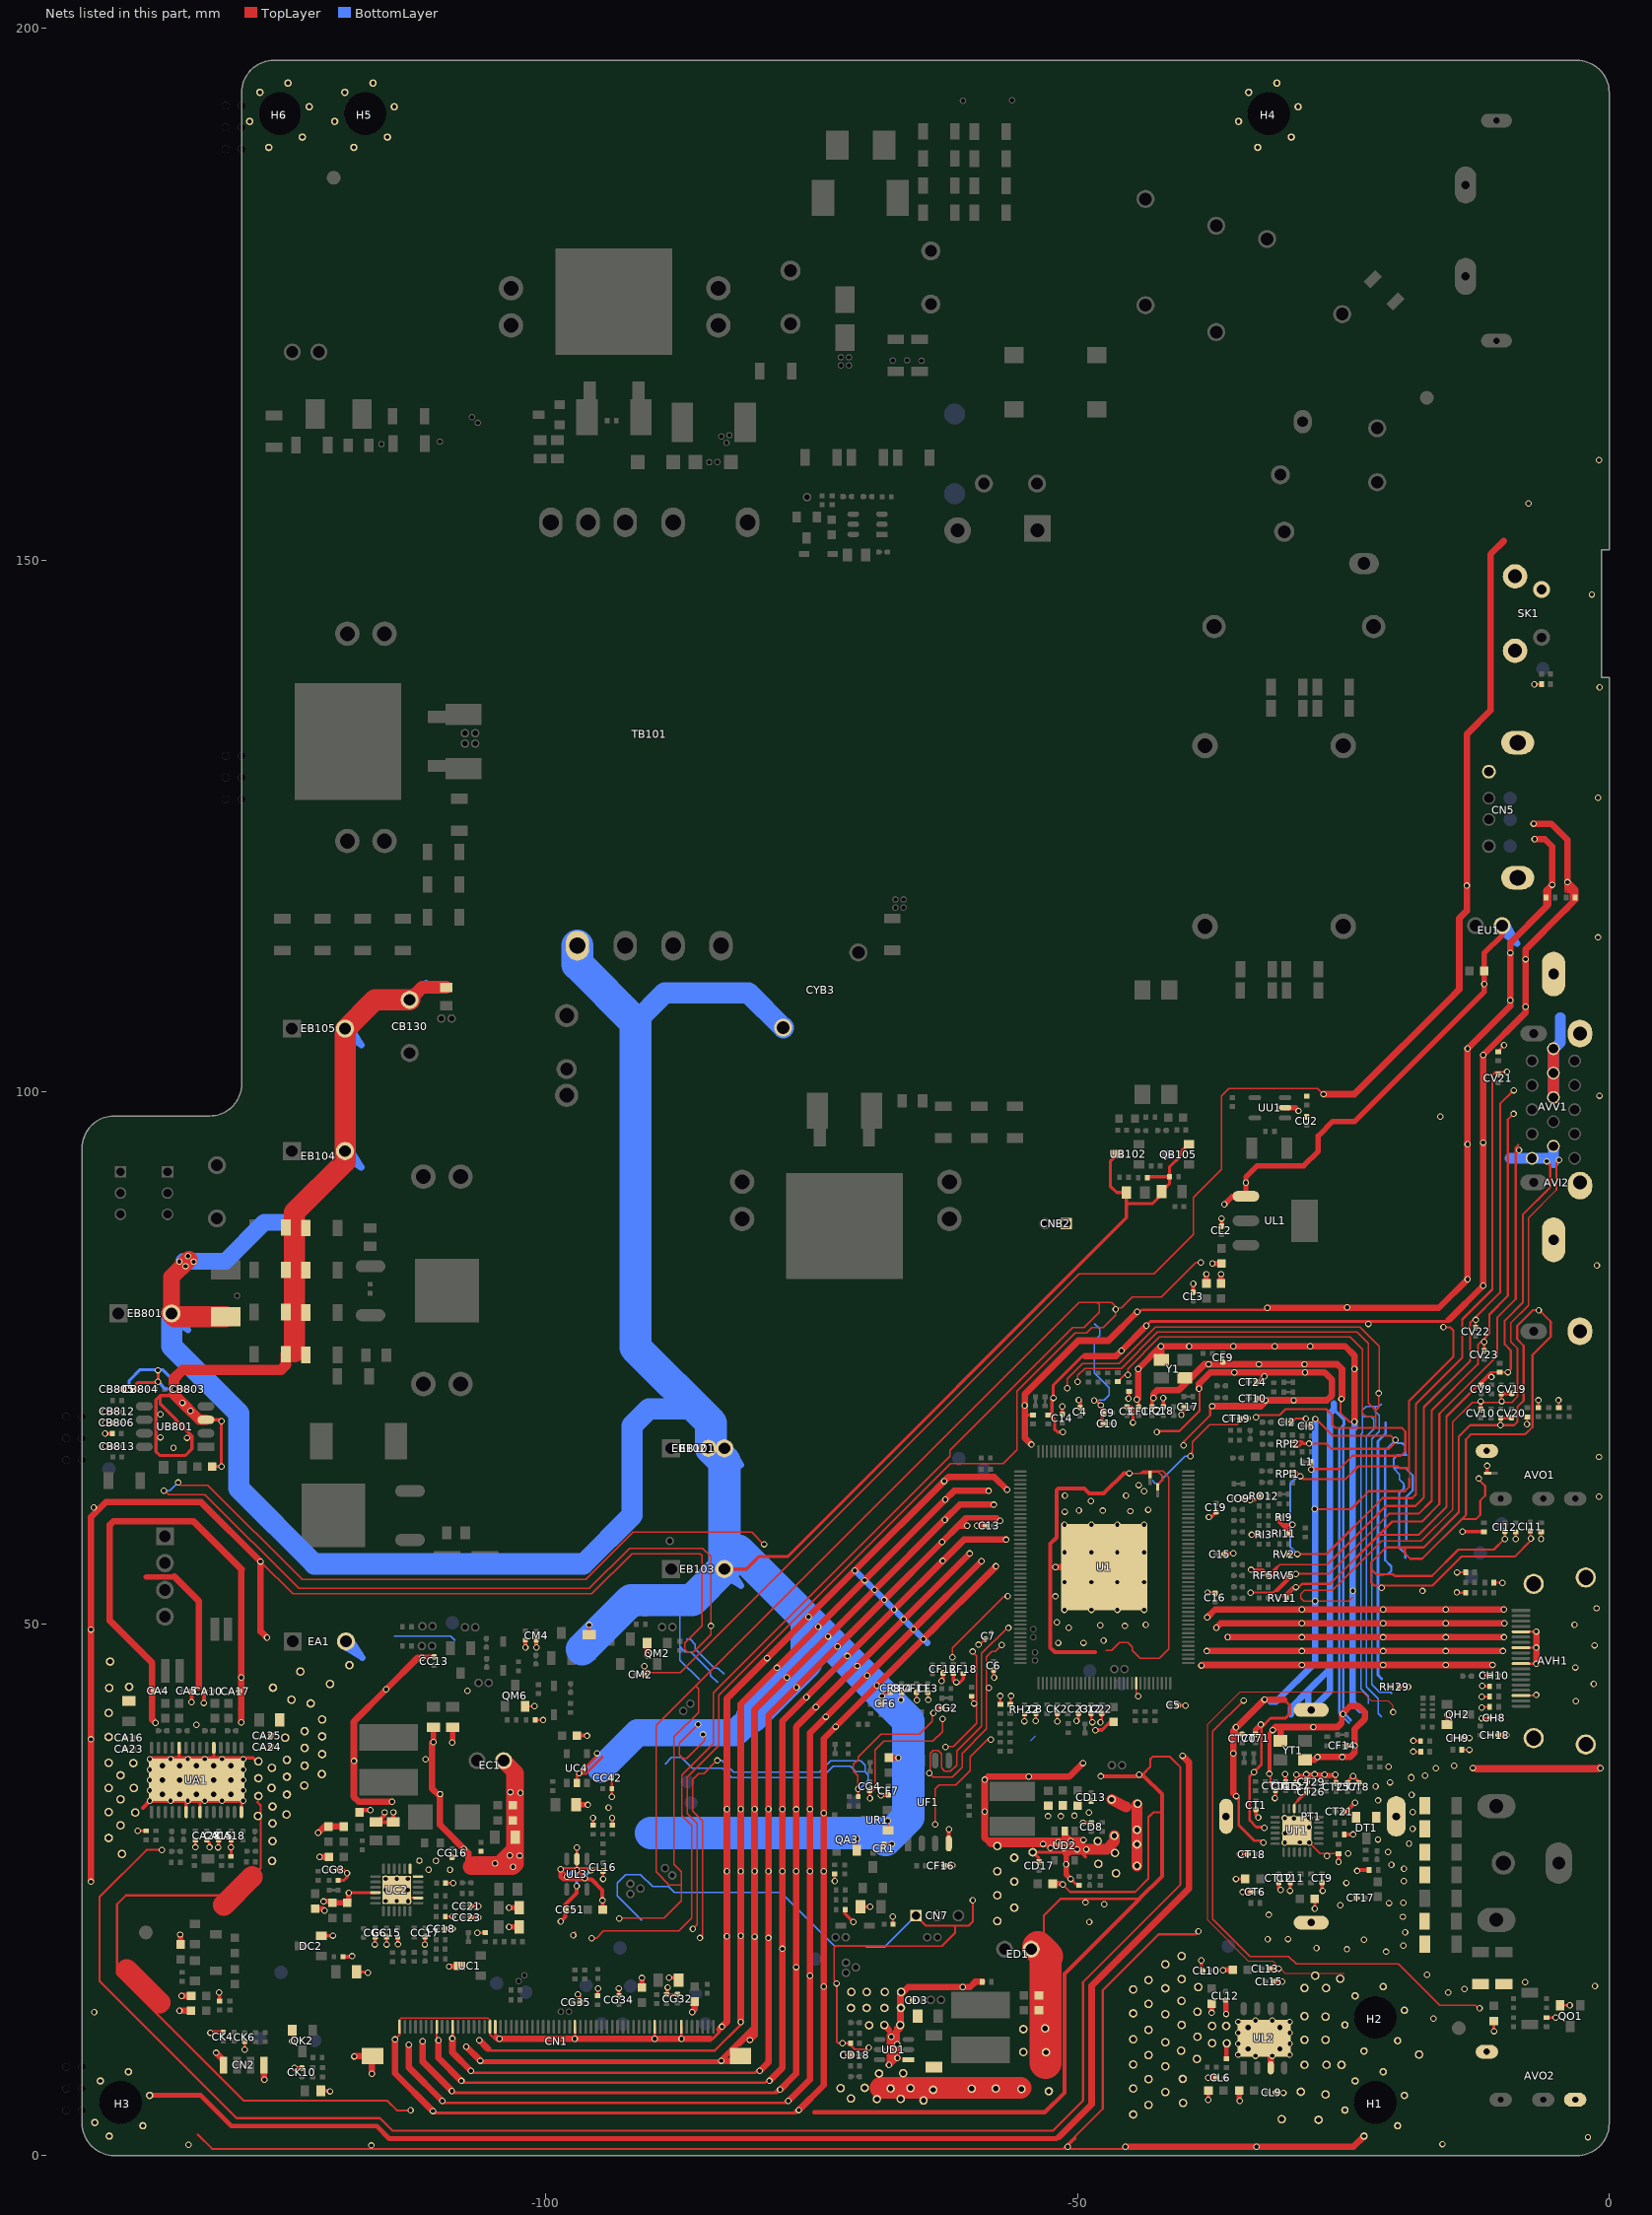
[diagram p0: the nets of this part, all layers, seen from the top]
# Altium PCB MISC86383-9.PcbDoc (part 11 of 18)
Units mm, origin at the board's own origin, x right, y up, seen from the top; angles counter-clockwise.
Board outline 143.6 x 197 mm, 2 copper layers (TopLayer, BottomLayer), stack 1.571 mm thick; 743 components, 401 nets, 2996 pads, 1077 vias.
Unrouted connection lines stored in the file: 4.

## Via types
v1: diameter 0.6, hole 0.4, TopLayer to BottomLayer, tented both sides, 993 vias
v2: diameter 0.6, hole 0.4, TopLayer to BottomLayer, 65 vias
v3: diameter 0.7, hole 0.5, TopLayer to BottomLayer, tented both sides, 15 vias
v4: diameter 0.8, hole 0.5, TopLayer to BottomLayer, tented both sides, 4 vias

## Nets (pads, with @x,y where several pads share a name; then routed paths per layer and width w, separated by ;. In a path a pad name is that pad's centre, name@x,y a point inside that pad or via, vN(x,y) a via of type N, cw(c..) or ccw(c..) an arc to the next point about the centre after c; other vN are vias at no path point) (continued)
GND: (continued)
  TopLayer w0.381: -137.877,32.7 -137.214,33.362 -133.82,33.362 -132.52,33.362 v1(-128.452,33.362) ; v1(-133.332,42.631) -133.314,42.65 CA5.2@-133.314,43.673 ; v1(-132.177,42.555) -132.157,42.574 CA10.2@-132.157,43.66 ; v1(-131.545,11.551) -131.497,11.599 CK4.2@-130.333,11.599 ; RC24.1@-119.082,18.694 -118.262,18.694 v1(-118.212,18.745) ; CG14.2@-117.5,32.266 -117.292,32.474 v1(-116.51,32.474) ; v1(-115.151,32.271) -115.151,32.017 -115.809,31.359 RG58.2@-115.976,31.359 RG63.2@-114.351,31.359 -114.351,32.042 -114.338,32.055 v1(-114.338,32.271) ; v1(-111.62,46.812) -111.513,46.92 CC13.1@-110.503,46.92 ; v1(-106.15,8.907) -106.036,8.793 -83.611,8.793 v1(-83.496,8.907) -81.912,10.491 ; v1(-101.917,47.765) RM6.2@-101.917,48.445 ; CM4.2@-100.902,48.444 -100.902,47.777 v1(-100.889,47.765) ; v1(-98.606,26.904) -98.606,26.205 -98.359,25.958 -95.688,25.958 -94.678,24.948 v1(-94.678,23.978) -94.678,23.939 -94.645,23.906 CC50.2@-94.645,23.114 ; v1(-98.59,22.009) -98.164,22.435 CC51.1@-98.164,23.114 -98.164,23.609 -97.097,24.676 v1(-97.097,25.353) ; CC38.1@-97.071,39.484 -96.152,39.484 v1(-96.126,39.459) ; -74.778,4.069 -53.065,4.069 -51.224,5.909 -51.224,17.087 -44.181,24.13 ; CF16.2@-62.458,27.254 -61.804,27.254 v1(-61.766,27.292) ; UF1.4@-62.106,29.342 -62.106,30.629 v1(-62.078,30.658) ; -48.355,47.327 -52.121,47.327 -52.546,47.752 -52.546,57.526 -51.964,58.108 -51.964,62.563 -51.797,62.729 -49.373,62.729 -48.888,62.244 -47.538,62.244 -45.63,64.152 v1(-45.109,64.152) ; v1(-47.803,35.662) -43.752,35.662 ; v1(-44.194,35.808) -43.899,35.808 -43.891,35.801 -43.752,35.662 ; -44.162,24.149 -42.056,26.255 -42.056,32.258 -42.056,33.965 -43.752,35.662 ; -43.415,35.325 -43.752,35.662 ; CL3.1@-39.116,81.197 v2(-39.116,81.966) ; v1(-37.719,7.315) CL6.1@-36.975,7.315 ; v1(-37.694,5.232) -37.689,5.237 CL7.1@-37.689,6.096 ; CL2.1@-36.449,87.416 v2(-36.449,88.113) ; RL4.1@-35.992,9.112 -35.992,10.515 pad.VIA5@-35.966,10.54 ; CT70.2@-34.55,39.66 CT70.2@-34.52,39.629 ; v2@-31.954,35.775 -31.954,39.703 v1(-31.65,40.007) ; CL15.2@-31.528,16.358 v1(-30.759,16.358) ; RI9.1@-31.002,59.921 -31.002,59.571 -30.633,59.203 ; v1@-30.915,24.976 v1@-30.871,24.932 ; RI11.1@-30.152,58.486 -30.152,58.721 -30.633,59.203 ; v1(-30.007,24.894) v1@-29.987,24.914 ; v1(-29.791,59.307) -30.529,59.307 -30.633,59.203 ; v1@-29.436,35.765 -29.368,35.698 v1@-28.451,35.698 ; CT29.1@-28.451,35.13 v1@-28.451,35.698 ; -26.26,35.666 -27.213,35.666 -27.245,35.698 -25.859,35.698 v1(-25.753,35.803) v1(-26.782,35.803) ; v1@-25.435,27.726 LT6.2@-25.435,28.393 ; v1@-25.327,23.564 -25.313,23.564 v1(-25.284,23.536) ; CT21.2@-24.947,32.348 -24.719,32.348 v1(-23.883,33.185) ; LT8.2@-24.921,30.177 v1@-24.089,30.177 ; CF14.1@-24.685,38.547 -23.954,38.547 v1(-23.941,38.534) ; v1(-23.695,26.761) -23.618,26.838 LT11.2@-22.571,26.838 ; v1@-1.155,83.62 v1(-1.155,83.679) ; v1@-0.973,65.633 -0.973,65.668 v1(-0.955,65.686) ; v1@-28.451,35.698 -27.958,35.698 -27.852,35.803 v1(-26.782,35.803) ; v1@-28.451,35.698 -28.451,35.822 v1(-28.471,35.841) v1(-27.696,35.841) -26.82,35.841 v1(-26.782,35.803)
  TopLayer w0.457: H3.4@-137.25,5.65 -132.445,5.65 -129.564,2.769 ; -128.727,2.769 -129.564,2.769 ; -51.675,1.906 -51.989,1.592 -114.725,1.592 -115.901,2.769 -129.564,2.769 ; -49.398,75.163 -49.29,75.163
  TopLayer w0.508: -137.594,54.421 -134.914,54.421 -134.125,53.632 ; v1(-134.379,20.777) -134.353,20.752 CG28.2@-134.353,19.845 ; CC5.2@-121.672,23.213 -121.015,23.213 v1(-120.82,23.017) ; v1@-120.905,23.877 v1(-120.905,23.886) -120.182,23.886 CC7.1@-120.053,23.757 CC4.2@-118.681,23.757 ; CC4.2@-118.686,23.762 CC4.2@-118.681,23.757 ; v1(-118.516,24.701) -118.516,23.922 CC4.2@-118.594,23.845 ; CC12.1@-110.582,40.253 -110.582,38.891 v1(-110.579,38.887) ; v1(-109.106,17.763) -109.034,17.763 -109.03,17.768 -108.179,17.768 UC1.3@-108.103,17.843 ; v1(-108.814,38.824) -108.75,38.824 -108.75,40.25 CC8.1@-108.753,40.253 ; v1@-103.454,21.483 CC1.1@-102.488,21.483 ; v1@-103.454,23.312 CC2.1@-102.488,23.312 ; CC43.1@-97.154,32.982 -96.05,32.982 v1(-96.037,32.969) ; CG33.1@-90.957,15.794 v1(-90.957,16.7) ; QM2.E@-90.475,48.197 -90.475,47.066 v1(-90.437,47.028) ; CF10.1@-67.755,37.41 -66.856,37.41 v1(-66.84,37.395) ; -60.533,59.893 -60.482,59.945 -57.604,59.945 -57.302,59.643 -57.252,59.643 v1(-57.252,59.69) ; CD16.1@-52.329,25.552 -51.46,25.552 v1(-51.384,25.476) ; v1(-50.648,26.01) -51.073,26.435 v1(-51.073,27.366) -51.073,28.402 -50.959,28.516 -50.936,28.538 -49.791,28.538 ; CL5.1@-37.871,82.004 v2(-37.871,82.88) ; v1(-37.389,13.411) CL11.2@-37.389,14.28 ; v2(-37.313,83.871) -37.308,83.876 CL1.1@-36.449,83.876 ; CL4.1@-36.5,82.004 v2(-36.5,82.88) ; v1(-36.322,17.424) -36.271,17.475 CL14.2@-35.403,17.475 ; v2(-36.195,89.433) -35.43,90.198 UL1.1@-34.163,90.198 v2(-34.163,91.491) -34.163,91.999 -33.096,93.066 -28.727,93.066 -27.356,94.437 -27.356,94.945 ; v1(-36.017,13.31) -36.017,14.28 ; -35.138,39.66 -35.138,40.144 v1@-35.138,40.214 ; v1@-35.092,40.342 v1(-35.092,40.26) ; CL8.1@-34.793,6.096 -34.793,5.177 v1(-34.747,5.131) ; CT71.1@-33.266,39.654 -33.266,40.045 -33.251,40.045 v1(-32.768,40.528) ; CL13.2@-31.884,17.577 v1(-31.09,17.577) ; UU1.2@-30.477,98.527 -29.515,98.527 v1(-29.21,98.222) ; -27.356,95.484 -27.356,94.945 ; -25.205,40.622 -25.154,40.672 -25.154,41.401 v1(-25.035,41.52) ; v2@-11.74,110.165 CU1.1@-11.74,111.379 ; EU1.2@-10.078,115.646 -10.078,114.737 -11.735,113.081 v2(-11.735,110.16) -11.735,109.436 -23.94,97.231 -25.997,97.231 -27.356,95.872 -27.356,94.945 ; -4.411,116.87 -4.376,116.87 -3.392,117.853 ; -4.411,116.871 -4.411,116.942 -3.392,117.961 DU4.A@-3.199,118.154 ; CC4.2@-118.681,23.757 CC4.2@-118.594,23.845 ; CC4.2@-118.681,23.757 -118.681,23.845 CC4.2@-118.594,23.845 ; v1@-35.138,40.214 v1(-35.092,40.26) ; v1@-35.138,40.214 -35.138,40.26 v1(-35.092,40.26)
  TopLayer w0.61: v1(-142.775,25.742) v1(-142.775,39.132) v1(-142.775,49.462) -142.775,60.033 -141.377,61.43 -132.41,61.43 v2(-126.835,55.854) -126.835,49.314 ; -140.997,51.15 -140.997,50.293 ; v1(-136.711,40.675) -137.015,40.98 -137.015,46.312 -140.997,50.293 ; -134.937,54.445 -134.914,54.421 -132.639,52.146 -132.639,44.044 ; v1(-134.455,13.614) CC34.1@-133.358,13.614 ; v1(-134.239,15.011) CC33.1@-133.345,15.011 ; v1(-131.009,9.659) -130.305,8.955 CN2.1@-130.305,8.505 CN2.1@-130.289,8.489 ; v1@-128.638,44.955 -128.638,48.59 ; -128.638,47.284 -128.638,48.59 ; v1(-128.633,40.739) v1(-128.633,44.955) ; -128.613,55.118 -129.673,56.178 ; -126.835,49.276 -126.835,49.314 ; CN2.4@-126.495,8.505 -126.495,7.153 v1(-126.467,7.125) ; v1(-126.213,48.692) -126.835,49.314 ; v1(-121.4,30.34) -120.807,30.932 CC10.2@-120.421,30.932 CC9.2@-118.999,30.932 ; v1(-121.26,28.08) -121.094,28.08 -121.082,28.092 CC11.2@-120.404,28.092 ; v1(-118.008,9.322) -117.978,9.353 CN1.62@-116.29,9.353 -116.357,9.285 v1(-116.357,7.671) ; v1(-114.449,33.261) -117.593,33.261 -118.046,33.715 v1(-118.046,37.097) -118.046,40.793 v1(-115.015,43.825) -112.028,46.812 v1(-111.62,46.812) ; v1(-114.173,10.909) v1(-114.173,10.909) -114.172,7.733 v1(-110.622,4.183) ; v1(-112.871,10.414) -112.871,8.272 v1(-109.727,5.128) ; v1(-111.571,10.757) -111.571,8.81 v1(-108.833,6.073) ; v1@-110.582,38.891 -110.718,38.755 -110.718,34.519 -109.969,33.77 -109.969,31.102 -107.29,28.423 -107.29,27.826 ; v1(-110.084,10.82) -110.084,9.162 v1(-107.939,7.018) ; v1@-108.783,11.024 v1(-108.783,11) -108.783,9.701 v1(-107.044,7.962) ; v1(-107.483,10.24) v1(-106.15,8.907) ; v1(-106.241,10.837) -105.432,10.028 ; -104.681,11.116 -104.537,10.973 v1(-104.343,10.973) v1(-97.282,10.973) v1(-89.764,10.973) v1(-87.236,10.973) -84.57,10.973 ; v1(-86.246,13.487) -85.992,13.741 CG31.1@-85.992,14.47 ; -83.693,11.85 v1(-83.431,12.112) -82.969,12.574 v1(-82.969,20.626) v1(-82.969,32.563) -82.969,42.978 v1(-70.931,55.016) v1(-62.535,63.412) -62.15,63.797 -57.816,63.797 v1(-56.624,62.604) ; v1(-83.496,8.907) -82.155,8.907 CN1.61@-81.71,9.353 ; -81.912,10.491 -80.368,12.036 ; v1(-81.668,12.548) v1(-81.668,20.656) -81.668,42.44 v1(-62.433,61.675) -61.611,62.496 v1(-58.355,62.496) ; v1(-80.823,10.858) -80.368,11.314 -80.368,12.036 ; -80.368,21.199 v1(-80.368,20.584) ; -80.368,24.028 -80.368,24.638 ; v1(-79.869,7.962) -79.425,8.407 -79.065,8.767 -79.065,11.716 v1(-79.065,20.455) ; -79.065,21.221 v1(-79.065,20.455) ; v1(-78.975,7.018) -78.785,7.208 -77.765,8.228 -77.765,12.436 ; v1(-77.967,6.187) -76.824,7.33 ; -77.765,13.462 -77.765,12.436 ; -77.765,21.391 v1(-77.765,19.435) ; -77.24,6.914 -76.824,7.33 ; v1@-77.059,5.255 -75.164,7.151 -75.164,17.424 ; -76.464,15.189 -76.464,13.371 ; -76.464,20.665 v1(-76.464,17.715) ; v1(-76.204,4.271) -73.863,6.612 -73.863,14.224 v1(-73.863,15.887) v1(-73.863,32.207) ; -75.164,16.561 v1(-75.164,16.903) -75.164,17.424 ; v1@-73.863,32.41 v1(-73.863,32.207) ; pad.VIA5@-68.17,12.263 -67.721,11.815 ; v1(-67.721,8.519) v1@-67.627,8.613 ; v1@-67.627,11.283 -67.627,10.333 v1@-67.627,8.613 ; v1@-67.618,9.862 v1(-67.607,9.862) ; -66.98,11.361 v1@-66.98,10.508 ; pad.VIA5@-66.624,12.192 -66.65,12.217 -66.65,15.113 -65.913,15.85 v1(-60.782,15.85) ; -63.267,49.803 v1(-64.498,48.572) ; -60.533,59.893 -61.22,59.207 ; v1(-60.361,59.207) -61.22,59.207 ; -60.316,15.826 -60.782,15.826 v1(-60.782,15.85) ; v1(-60.143,56.606) v1(-66.338,50.41) -76.464,40.284 v1(-76.464,17.715) ; v1(-59.02,55.889) v1(-65.41,49.499) -75.164,39.745 -75.164,17.424 ; DK6.A@-58.947,16.332 -59.607,16.332 -60.09,15.85 v1(-60.782,15.85) ; v1(-57.872,61.196) -61.073,61.196 v1(-62.477,59.792) v1(-69.085,53.183) -80.368,41.901 -80.368,24.638 ; v1(-57.667,55.403) v1(-64.498,48.572) ; v1(-56.703,57.906) -60.681,57.906 v1(-62.672,55.916) v1(-67.246,51.341) -77.765,40.823 v1(-77.765,19.435) ; v1(-54.331,66.853) -54.966,67.488 -54.966,69.716 v1(-54.966,70.529) -54.966,71.577 -49.922,76.621 -47.085,76.621 v1(-44.378,79.328) ; v1(-52.07,55.321) -52.062,55.313 U1.157@-47.471,55.313 ; v1(-51.821,29.464) -51.821,29.396 v1@-51.918,29.299 ; -51.731,1.754 -48.672,4.814 -48.672,15.964 -39.503,25.132 -39.503,36.963 v1(-40.132,37.592) ; v1(-51.308,28.905) v1(-50.648,29.566) ; UD2.2@-51.199,30.507 UD2.2@-51.199,30.117 ; v1(-50.038,28.792) v1@-50.038,28.956 ; v1(-49.484,36.898) -50.758,35.623 v1(-54.585,35.623) -58.434,35.623 v1(-58.725,35.332) v1(-58.725,32.334) -58.725,29.867 -58.46,29.603 ; -49.29,75.163 -46.391,75.163 v1(-45.872,75.682) v1(-43.525,78.029) ; v1(-45.494,0.826) v1(-33.172,0.826) -24.049,0.826 H1.6@-23.05,1.825 ; v1(-44.425,71.082) -44.278,71.229 v1@-44.278,73.938 ; v1(-44.296,73.956) v1(-42.168,76.084) v1(-39.497,76.084) v1(-35.344,76.084) v1(-31.458,76.084) v1(-28.118,76.084) -24.814,76.084 -23.96,75.23 v1(-23.96,73.97) v1(-23.96,68.991) ; v1(-42.848,71.213) -42.848,71.607 -42.47,71.985 -40.475,71.985 -38.06,74.401 v1(-37.653,74.401) v1(-32.941,74.401) v1(-28.651,74.401) -25.569,74.401 -25.128,73.959 -25.128,71.2 v1(-25.179,71.15) ; v1@-42.15,76.066 -42.106,76.022 Y1.2@-42.106,74.82 ; v1(-38.568,72.115) -38.568,72.572 -37.501,73.639 v1(-35.255,73.639) v1(-28.602,73.639) -26.75,73.639 -26.06,72.949 -26.06,71.485 -26.53,71.015 v1(-29.667,71.015) v1(-32.343,71.015) -32.343,70.86 -32.744,70.459 v1(-37.327,70.459) ; v1(-38.34,46.079) -38.29,46.129 v1(-28.906,46.129) v1(-21.26,46.129) v1(-15.354,46.129) v1(-10.97,46.129) ; v1(-37.851,47.429) v1(-28.906,47.429) v1(-21.26,47.429) v1(-15.354,47.429) v1(-9.982,47.429) ; v1(-37.814,50.589) -37.066,51.337 v1(-28.906,51.337) v1(-9.892,51.337) ; v1(-36.943,49.622) -36.528,50.037 v1(-28.906,50.037) v1(-21.26,50.037) v1(-15.354,50.037) v1(-9.853,50.037) ; v1(-35.877,48.736) -35.871,48.73 v1(-28.906,48.73) v1(-21.26,48.73) v1(-15.354,48.73) v1(-9.884,48.73) ; v1@-35.138,33.855 -35.352,34.07 -35.352,39.929 -35.138,40.144 v1(-32.404,42.878) -30.574,42.878 ; UL2.EPAD@-32.461,11.024 -31.826,10.389 UL2.3@-31.826,8.241 ; v2(-32.155,79.705) -23.546,79.705 ; v1(-31.65,40.007) -31.369,40.289 v1(-27.815,40.289) -25.537,40.289 -25.205,40.622 ; YT1.4@-30.908,39.002 -30.908,40.18 ; YT1.2@-28.608,37.202 -27.699,37.202 v1(-27.434,37.467) v1(-25.11,37.467) -24.36,37.467 -23.941,37.886 v1(-23.941,38.534) -23.941,40.096 -22.951,41.087 -22.952,41.088 -22.952,41.652 -23.557,42.257 -24.362,42.257 v1@-25.035,41.585 ; v2(-26.873,99.797) -23.96,99.797 -14.723,109.034 ; v1@-25.154,41.401 -25.154,41.466 v1@-25.035,41.585 ; v1(-25.035,41.52) v1@-25.035,41.585 ; v1(-24.638,79.756) -24.587,79.705 -23.546,79.705 ; -15.076,78.577 v1(-11.854,81.799) v1(-11.854,95.25) v1(-11.854,103.475) -7.847,107.481 v1(-7.847,108.024) v1(-7.847,112.493) -7.847,113.398 ; -14.503,109.254 -14.723,109.034 ; -13.995,116.434 -13.392,117.037 ; v2(-13.392,119.405) -13.392,123.215 ; v1(-12.827,36.436) v1@-0.851,36.436 ; CN5.4@-11.31,129.959 CN5.4@-11.31,130.13 ; -9.922,151.807 -11.144,150.585 -11.144,135.889 -13.392,133.641 -13.392,123.215 ; v1(-7.102,125.238) -5.452,125.238 -3.907,123.693 v1(-3.907,119.732) ; v1(-7.007,123.78) -6.056,123.78 -5.365,123.089 v1(-5.365,119.487) -5.736,119.116 ; v1(-6.858,46.228) v1(-6.858,47.752) v1(-6.858,49.276) ; -4.376,116.87 -7.847,113.398 ; -3.864,117.417 -4.097,117.184 ; -3.392,117.961 -3.392,118.761 -3.907,119.275 v1(-3.907,119.732) ; v1@-0.945,36.53 v1@-0.851,36.436 ; v1(-0.826,36.411) v1@-0.851,36.436 ; -140.997,50.293 -140.997,59.296 -140.641,59.652 -133.147,59.652 -129.673,56.178 ; -129.673,56.178 -128.638,55.143 -128.638,48.59 ; -80.368,12.036 -80.368,12.497 v1(-80.368,20.584) ; v1(-80.368,20.584) -80.368,24.638 ; v1(-79.065,20.455) -79.065,41.361 v1(-68.175,52.253) v1(-62.728,57.699) -61.22,59.207 ; -77.765,12.436 v1(-77.765,19.435) ; -76.824,7.33 -76.464,7.689 -76.464,13.371 ; -76.464,13.371 v1(-76.464,17.715) ; v1(-73.863,32.207) -73.863,39.207 v1(-64.498,48.572) ; v1@-67.627,8.613 -67.074,9.166 v1(-66.933,9.166) v1@-66.98,9.213 ; v1(-67.607,9.862) -67.552,9.862 v1@-66.98,10.434 ; v1(-67.607,9.862) -67.607,9.84 v1@-66.98,9.213 ; v1@-66.98,9.213 v1@-66.98,10.434 ; v1@-66.98,10.434 v1@-66.98,10.508 ; v1@-66.98,10.434 v1(-66.943,10.471) v1@-66.98,10.508 ; v1@-66.98,10.508 -67.505,11.034 v1(-67.505,11.157) -66.933,11.73 ; -66.933,11.73 -66.933,11.993 pad.VIA5@-66.663,12.263 -66.663,12 -66.933,11.73 ; -58.46,29.603 -51.257,29.603 ; -58.46,29.603 -58.156,29.299 v1(-53.238,29.299) v1@-51.918,29.299 ; v1@-51.918,29.299 -51.561,29.299 -51.257,29.603 ; -51.257,29.603 -51.199,29.661 ; -51.199,29.661 UD2.2@-51.199,30.117 ; -51.199,29.661 -51.193,29.667 v1@-50.749,29.667 ; UD2.2@-51.199,30.117 v1@-50.749,29.667 ; v1@-50.749,29.667 v1(-49.428,29.667) -50.038,29.058 v1@-50.038,28.956 ; v1@-50.749,29.667 v1(-50.648,29.566) ; v1(-50.648,29.566) v1@-50.038,28.956 ; -23.546,79.705 -16.01,79.705 v1(-13.312,82.403) v1(-13.312,95.098) v1(-13.312,104.078) -9.305,108.085 v1(-9.305,108.628) v1(-9.305,113.097) -9.305,114.037 -5.929,117.413 ; -14.723,109.034 -14.092,109.665 -14.092,116.337 -13.392,117.037 ; -13.392,117.037 -13.392,123.215 ; -7.847,113.398 -7.847,113.433 ; -7.847,113.433 -4.411,116.87 -4.097,117.184 ; -7.847,113.434 -4.411,116.871 -4.097,117.184 ; -5.929,117.413 DU3.A@-5.929,118.305 -5.925,118.309 -5.925,118.927 -5.736,119.116 ; -5.929,117.413 -5.736,117.607 -5.736,119.116 ; -4.097,117.184 -3.199,118.082 -3.199,118.154 DU4.A@-3.199,118.307 -3.199,119.025 v1(-3.907,119.732)
  TopLayer w1: v2(-133.427,70.027) -132.95,69.551 ; UB801.3@-131.961,69.18 -132.58,69.18 -132.95,69.551 ; RB839.2@-124.446,75.349 -124.446,74.347 -124.917,73.876 -134.158,73.876 -134.975,73.059 -134.975,71.576 v2(-134.176,70.777) -132.95,69.551
  TopLayer w1.016: -51.001,28.603 -50.812,28.792 v1(-50.038,28.792) v1(-49.174,28.792) -47.249,28.792 -46.519,29.523 pad.VIA5@-46.533,30.074 ; pad.VIA5@-46.787,33.477 -45.431,32.766 ; pad.VIA5@-44.405,27.228 pad.VIA5@-44.405,29.26 pad.VIA5@-44.405,32.994 ; AVV1.8@-5.247,99.595 AVV1.7@-5.247,101.785 AVV1.6@-5.247,104.075 AVV1.6@-5.247,104.175
  TopLayer w1.2: CB130.1@-112.812,108.661 -111.629,109.845 RB140.2@-109.36,109.845
  TopLayer w1.524: -107.038,27.14 -104.623,27.14 ; -106.718,27.368 -104.394,27.368 ; -104.369,27.368 -104.394,27.368 ; EC1.2@-103.969,37.122 -102.946,36.099 ; -104.623,27.14 pad.VIA5@-103.083,27.14 -102.806,27.417 -102.806,28.956 ; -104.623,27.14 -104.394,27.368 ; -104.394,27.368 -102.946,28.816 ; -102.946,28.816 -102.946,36.099 ; -102.946,28.816 -102.806,28.956 ; -102.946,36.099 -102.806,35.959 -102.806,28.956
  TopLayer w1.6: EB801.2@-135.193,79.184 -135.193,82.599 -133.547,84.245
  TopLayer w2: EB801.2@-135.193,79.184 -134.873,78.864 DB804.K@-130.111,78.864 ; -123.622,75.578 -123.622,88.697 -118.874,93.445 EB104.2@-118.874,94.45 -118.874,105.865 -116.078,108.661 CB130.1@-112.812,108.661
  TopLayer w2.032: -139.396,17.446 -136.324,14.374 ; -130.273,23.546 -130.282,23.546 -127.618,26.209 ; -68.529,6.375 pad.VIA5@-55.334,6.375
  TopLayer w3: ED1.2@-53.726,19.601 -52.996,18.871 ; -52.996,8.714 -52.996,18.871 ; -52.856,18.731 -52.996,18.871
  BottomLayer w0.102: -54.394,39.017 -53.926,39.486
  BottomLayer w0.127: v2(-135.903,62.522) -135.344,62.522 v2(-134.582,63.284) ; -114.267,48.852 -108.948,48.852 -108.509,48.412 ; -90.946,22.084 -93.256,24.393 -93.256,25.627 -92.467,26.416 -91.084,26.416 -89.952,25.284 -88.46,25.284 -87.903,24.727 -77.876,24.727 -72.834,19.685 -69.124,19.685 -69.086,19.647 ; -88.794,36.792 -88.163,37.422 -87.262,37.422 -86.238,36.398 -83.42,36.398 -82.548,35.527 -74.062,35.527 -72.98,36.609 -71.369,36.609 -70.836,36.076 -69.964,36.076 ; -87.404,47.844 -86.923,47.363 -86.381,47.363 -84.501,45.483 -84.501,45.149 -83.845,44.492 ; -86.786,48.54 -86.429,48.54 -85.946,48.057 -85.946,47.646 -84.142,45.842 -83.807,45.842 -83.216,45.251 ; -86.248,52.222 -87.37,51.1 -87.37,46.59 -85.56,44.78 ; v1@-84.066,37.143 -83.446,37.143 -82.338,36.035 -74.273,36.035 -73.19,37.117 -70.366,37.117 -69.964,36.716 -69.964,36.076 ; v1(-70.637,34.468) -70.46,34.468 -69.677,35.25 -69.677,35.789 -69.964,36.076 ; -48.396,78.228 -47.904,77.737 -47.904,77.114 -48.435,76.584 -48.435,73.595 -47.031,72.191 -47.031,71.511 -47.503,71.04 -48.009,71.04 ; -42.954,63.462 -42.717,63.225 -42.331,63.225 -42.059,63.498 -42.059,63.58 -39.878,65.761 v1(-39.383,65.761) ; v1(-23.96,68.991) -23.96,70.362 ; -22.657,42.486 -22.657,43.182 -23.359,43.884 -23.359,61.955 -23.359,67.098 -23.355,67.103 -23.355,67.796 -23.185,67.966 -23.185,69.435 ; -21.412,70.675 -21.654,70.434 -21.978,70.434 ; -21.386,41.247 -21.714,41.575 -21.714,42.957 -22.83,44.073 -22.83,67.603 -22.136,68.296 -22.136,69.219 -22.36,69.443 -23.178,69.443 -23.185,69.435 ; -20.401,43.41 -20.542,43.552 -21.59,43.552 -22.322,44.283 -22.322,67.392 -21.628,68.086 -21.628,69.58 -21.978,69.93 -21.978,70.434 ; -20.252,64.727 -20.252,64.59 -19.715,64.054 -19.715,63.567 -19.313,63.165 -19.313,62.992 ; -23.185,69.435 -23.185,70.091 -22.842,70.434 -21.978,70.434
  BottomLayer w0.203: -69.85,19.647 -69.086,19.647 -68.104,19.647 CN7.1@-65.195,22.555 ; v1(-29.307,56.552) -30.001,57.245 -30.001,63.151 -29.281,63.871 v1(-29.053,63.871) ; -25.062,68.581 -25.379,68.264 -25.379,41.566 -24.463,40.651 ; -21.214,54.632 -21.188,54.657 -20.807,54.657 -20.498,54.967 -20.498,55.405 -21.065,55.971 -21.065,66.298 v1(-20.087,67.276) ; -20.252,64.727 -20.252,65.523 -19.909,65.866 -19.045,65.866 ; -20.218,64.656 -19.181,64.656 -18.479,63.953 -18.479,62.529 -19.083,61.924 -19.083,57.95 ; -19.912,66.979 -19.474,66.979 -19.164,66.67 -19.164,65.96 ; -19.313,62.992 -19.313,62.727 -19.744,62.296 -19.744,57.158 -19.177,56.591 -19.177,56.197
  BottomLayer w0.254: v1(-97.996,26.227) -97.4,26.823 v1(-97.068,26.823) -97.097,26.794 v1(-97.097,25.353) ; v1(-96.343,26.085) -96.343,26.22 v1(-95.761,26.802) ; -24.998,42.745 -24.998,43.275 ; -24.93,68.713 -24.998,68.645 -24.998,68.241 -24.998,43.275 ; -24.308,40.932 -24.998,41.622 -24.998,43.275 ; v1@-21.598,53.382 v1(-21.395,53.382) ; -21.598,54.665 -21.565,54.632 -21.214,54.632 ; -21.399,44.831 -21.75,45.182 -21.75,67.156 -21.014,67.892 -21.014,68.897
  BottomLayer w0.3: v2(-141.453,67.894) v2@-141.44,67.894 ; v2@-141.427,66.891 v2@-141.414,66.878 ; v2(-139.179,72.047) -139.179,72.873 -138.158,73.894 -136.518,73.894 v2(-136.461,73.838) ; v2(-136.461,73.838) -136.461,73.901 -136.042,73.901 -134.901,72.76 v2(-134.901,72.074) -135.765,72.074 -136.436,72.746 v2(-136.461,72.746) v2(-136.461,73.838)
  BottomLayer w0.305: -25.908,70.123 -25.86,70.123 -24.93,69.192 -24.93,68.713 ; -25.062,68.581 -24.998,68.645
  BottomLayer w0.61: v1(-70.931,55.016) v1(-70.011,54.097) -64.131,48.217 ; -31.865,42.695 -31.307,42.695 -27.639,46.363 -27.639,47.548 ; -29.915,41.455 -29.915,42.111 -28.313,43.713 ; -27.639,46.803 v1@-27.639,69.24 ; -26.242,45.784 -28.313,43.713 ; -25.908,70.729 -25.908,70.123 -26.242,69.788 -26.242,43.681 PT1.3@-28.026,41.897 -28.313,42.184 -28.313,43.713 ; v1(-23.96,68.991) -23.935,68.965 -23.935,68.415 -24.109,68.241 -24.109,68.055 -24.109,67.613 -24.109,42.591 -23.426,41.908
  BottomLayer w1.016: -9.328,93.77 AVV1.5@-7.247,93.77 -5.683,93.77 ; -5.247,93.334 AVV1.10@-5.247,94.915 ; AVV1.8@-5.247,99.495 AVV1.7@-5.247,101.785 -5.247,103.996 -4.58,104.663 -4.58,107.004
  BottomLayer w1.6: -134.037,84.092 -130.119,84.092 -126.454,87.757 -123.469,87.757
  BottomLayer w2: EB801.2@-135.193,79.184 -135.193,76.1 -128.867,69.774 -128.867,62.738 -121.755,55.626 -96.456,55.626 -91.884,60.198 -91.884,68.631 -90.322,70.193 -85.776,70.193 -85.395,69.812 ; -91.567,106.566 -88.824,109.309 -80.934,109.309 CYB3.2@-77.678,106.053
  BottomLayer w2.54: -94.805,36.322 -91.389,39.738 -82.131,39.738 -80.594,41.275
  BottomLayer w3: TB101.7@-97.028,113.767 -97.028,112.027 -91.567,106.566 -91.567,75.984 -84.458,68.875 -84.458,66.521 -83.212,65.275
  BottomLayer w3.048: -96.577,47.619 -91.973,52.222 -86.248,52.222 EB103.2@-83.25,55.22 ; -90.119,30.328 -68.732,30.328 -68.059,29.654 -65.9,31.813 -65.9,40.869 v1@-75.476,50.444 ; EB102.2@-84.434,66.497 -83.212,65.275 EB103.2@-83.212,55.143 ; -80.594,41.275 -75.476,46.393 v1@-75.476,50.444 ; -81.928,56.896 v1@-75.476,50.444 ; -81.928,56.896 -83.149,56.896 -81.928,56.896